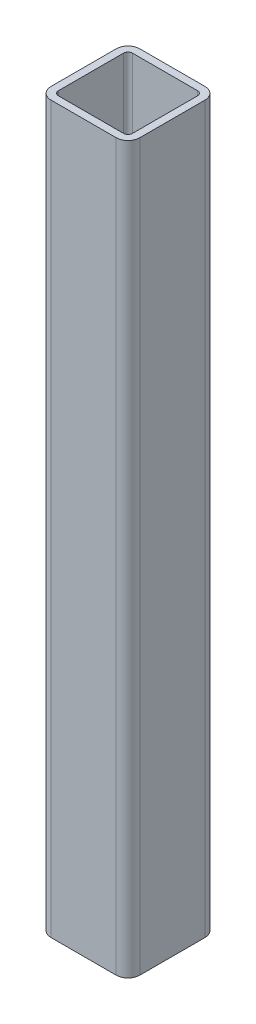
from build123d import *

# Parameters (mm, degrees)
GB_T6728_2002_120_120_10_1_DEPTH = 980


with BuildPart() as part:
    # Sketch12 → 结构用冷弯空心方钢(gb t6728-2002) 120×120×10(1) (new body)
    with BuildSketch(Plane(origin=(0, 0, 0), x_dir=(-1, 0, 0), z_dir=(0, 1, 0))):
        with BuildLine():
            Line((-44, -60), (44, -60))
            ThreePointArc((44, -60), (55.313708499, -55.313708499), (60, -44))
            Line((60, -44), (60, 44))
            ThreePointArc((60, 44), (55.313708499, 55.313708499), (44, 60))
            Line((44, 60), (-44, 60))
            ThreePointArc((-44, 60), (-55.313708499, 55.313708499), (-60, 44))
            Line((-60, 44), (-60, -44))
            ThreePointArc((-60, -44), (-55.313708499, -55.313708499), (-44, -60))
        make_face()
        with BuildLine():
            Line((-44, -50), (44, -50))
            ThreePointArc((44, -50), (48.242640687, -48.242640687), (50, -44))
            Line((50, -44), (50, 44))
            ThreePointArc((50, 44), (48.242640687, 48.242640687), (44, 50))
            Line((44, 50), (-44, 50))
            ThreePointArc((-44, 50), (-48.242640687, 48.242640687), (-50, 44))
            Line((-50, 44), (-50, -44))
            ThreePointArc((-50, -44), (-48.242640687, -48.242640687), (-44, -50))
        make_face(mode=Mode.SUBTRACT)
    extrude(amount=GB_T6728_2002_120_120_10_1_DEPTH)


solid = part.part
